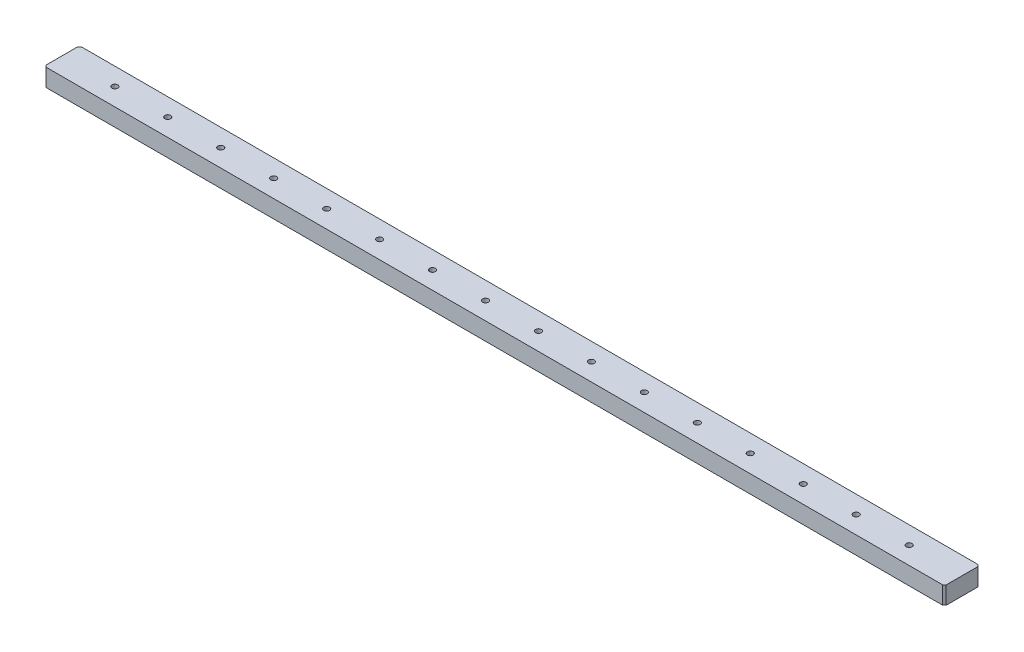
SolidWorks part; units mm, degrees
ref_plane "前视基准面" through (0, 0, 0) normal (0, 0, 1) x (1, 0, 0)
ref_plane "上视基准面" through (0, 0, 0) normal (0, 1, 0) x (1, 0, 0)
ref_plane "右视基准面" through (0, 0, 0) normal (1, 0, 0) x (0, 0, -1)
sketch "草图1" plane through (0, 0, 0) normal (0, 1, 0) x (1, 0, 0)
  line L1 (-510, -20) -> (510, -20)
  line L2 (-510, -20) -> (-510, 20)
  line L3 (-510, 20) -> (510, 20)
  line L4 (510, -20) -> (510, 20)
  line L5 (-510, -20) -> (510, 20) construction
  line L6 (-510, 20) -> (510, -20) construction
  point P0 (0, 0)
  dimension "D1" = 40
  dimension "D2" = 1020
extrude "凸台-拉伸1" add sketch "草图1" along normal blind 20
chamfer "倒角1" distance 2 angle 45 4 edges at (510, 10, 20) (-510, 10, 20) (-510, 10, -20) (510, 10, -20)
sketch "草图7" plane through (0, 0, 0) normal (0, -1, 0) x (-1, 0, 0)
  line L0 (510, 0) -> (452.0072, 0) construction
  line L1 (510, 18) -> (510, -18) construction
  line L3 (0, -20) -> (0, 57.4964) construction
  line L4 (508, -20) -> (-508, -20) construction
  line L6 (-510, 0) -> (-452.0072, 0) construction
  point P0 (480, -9.5)
  point P18 (-480, -9.5)
  dimension "D1" = 9.5
  dimension "D2" = 30
hole_wizard "Ø4.0mm 暗销孔1" positions "草图7" profile "草图6" hole size "Ø4.0" standard "GB"
sketch "草图6" plane through (-480, 0, 9.5) normal (1, 0, 0) x (0, 0, -1)
  line L0 (0, 0) -> (0, 13.2017)
  line L1 (0, 13.2017) -> (2, 12)
  line L2 (2, 12) -> (2, 0)
  line L5 (2, 0) -> (0, 0)
  line L10 (0, 13.2017) -> (-2, 12) construction
  line L11 (0, -6.35) -> (0, 107.95) construction
  dimension "孔直径" = 4
  dimension "孔深度" = 12
  dimension "导头角度" = 118
sketch "草图10" plane through (0, 0, 0) normal (0, -1, 0) x (-1, 0, 0)
  point P0 (-480, 0)
hole_wizard "M3 螺纹孔1" positions "草图10" profile "草图9" tap size "M3" standard "GB"
sketch "草图9" plane through (480, 0, 0) normal (1, 0, 0) x (0, 0, -1)
  line L0 (0, 0) -> (0, 8.2511)
  line L1 (0, 8.2511) -> (1.25, 7.5)
  line L2 (1.25, 7.5) -> (1.25, 0)
  line L5 (1.25, 0) -> (0, 0)
  line L10 (0, 8.2511) -> (-1.25, 7.5) construction
  line L11 (0, -6.35) -> (0, 107.95) construction
  dimension "螺纹孔钻头直径" = 2.5
  dimension "螺纹孔钻头深度" = 7.5
  dimension "导头角度" = 118
cosmetic thread "孔螺纹线1" parameters "D1"=6, "D2"=3
pattern_linear "阵列(线性)5" count 17 spacing 60 along (-1, 0, 0) of "M3 螺纹孔1"
sketch "草图4" plane through (0, 0, 0) normal (0, -1, 0) x (-1, 0, 0)
  line L0 (-510, -18) -> (-510, 18) construction
  point P0 (-450, 0)
  point P6 (-510, 0)
  dimension "D1" = 30
hole_wizard "M6 六角圆柱头螺钉的柱形沉头孔1" positions "草图4" profile "草图3" counterbore size "M6" standard "GB" end condition up to next
sketch "草图3" plane through (450, 0, 0) normal (1, 0, 0) x (0, 0, -1)
  line L0 (0, 0) -> (0, 20)
  line L1 (0, 20) -> (3.3, 20)
  line L3 (3.3, 20) -> (3.3, 6.8)
  line L4 (3.3, 6.8) -> (5.5, 6.8)
  line L5 (5.5, 6.8) -> (5.5, 0)
  line L7 (5.5, 0) -> (0, 0)
  line L11 (0, -6.35) -> (0, 107.95) construction
  dimension "通孔孔直径" = 6.6
  dimension "通孔孔深度" = 20
  dimension "柱形沉头孔直径" = 11
  dimension "柱形沉头孔深度" = 6.8
pattern_linear "阵列(线性)6" count 16 spacing 60 along (-1, 0, 0) of "M6 六角圆柱头螺钉的柱形沉头孔1"
